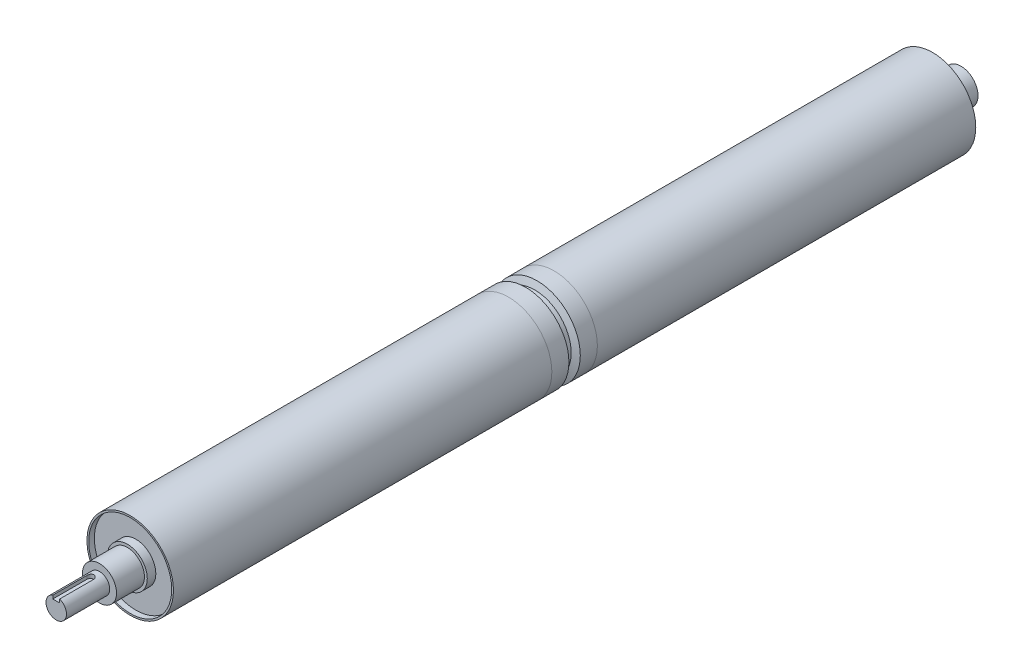
SolidWorks part; units mm, degrees
material "普通碳钢"
ref_plane "前视基准面" through (0, 0, 0) normal (0, 0, 1) x (1, 0, 0)
ref_plane "上视基准面" through (0, 0, 0) normal (0, 1, 0) x (1, 0, 0)
ref_plane "右视基准面" through (0, 0, 0) normal (1, 0, 0) x (0, 0, -1)
sketch "草图1" plane through (0, 0, 0) normal (0, 0, 1) x (1, 0, 0)
  circle A0 centre (0, 0) radius 38
  circle A1 centre (0, 0) radius 36.5
  dimension "D1" = 76
  dimension "D2" = 1.5
extrude "凸台-拉伸1" add sketch "草图1" along normal mid plane 705
sketch "草图2" plane through (0, 0, 352.5) normal (0, 0, 1) x (1, 0, 0)
  circle A1 centre (0, 0) radius 36.5 construction
  circle A2 centre (0, 0) radius 36.5
  circle A3 centre (0, 0) radius 17.5
  dimension "D1" = 35
extrude "凸台-拉伸2" add sketch "草图2" against normal blind 10 from offset 5 separate body offset against normal yes
sketch "草图3" plane through (0, 0, -352.5) normal (0, 0, -1) x (-1, 0, 0)
  circle A1 centre (0, 0) radius 17.5
  circle A2 centre (0, 0) radius 17.5
  circle A3 centre (0, 0) radius 36.5
  circle A4 centre (0, 0) radius 36.5
  dimension "D1" = 0
  dimension "D2" = 0
extrude "凸台-拉伸3" add sketch "草图3" against normal blind 10 from offset 5 separate body offset against normal yes
sketch "草图10" plane through (0, 0, 0) normal (0, 0, 1) x (1, 0, 0)
  circle A0 centre (0, 0) radius 17.5
  dimension "D1" = 35
extrude "凸台-拉伸4" add sketch "草图10" along normal mid plane 755 separate body
sketch "草图11" plane through (0, 0, 377.5) normal (0, 0, 1) x (1, 0, 0)
  circle A1 centre (0, 0) radius 17.5
  circle A2 centre (0, 0) radius 17.5
  dimension "D1" = 0
extrude "凸台-拉伸5" add sketch "草图11" along normal blind 40
sketch "草图15" plane through (0, 0, 417.5) normal (0, 0, 1) x (1, 0, 0)
  circle A0 centre (0, 0) radius 23.9517
  circle A1 centre (0, 0) radius 15
  dimension "D1" = 30
extrude "切除-拉伸2" cut sketch "草图15" against normal blind 62.5
sketch "草图16" plane through (0, 0, -377.5) normal (0, 0, -1) x (-1, 0, 0)
  circle A0 centre (0, 0) radius 15
  circle A1 centre (0, 0) radius 17.5 construction
  circle A2 centre (0, 0) radius 17.5
  dimension "D1" = 30
extrude "切除-拉伸3" cut sketch "草图16" against normal blind 22.5
sketch "草图18" plane through (0, 0, 0) normal (0, 0, 1) x (1, 0, 0)
  circle A0 centre (0, 0) radius 54.9628
  circle A1 centre (0, 0) radius 24.0057
extrude "切除-拉伸4" cut sketch "草图18" against normal mid plane 40
sketch "草图19" plane through (0, 0, 0) normal (0, 1, 0) x (1, 0, 0)
  line L0 (0, 0) -> (-63.5289, 0) construction
  line L1 (-36.5, 30) -> (-36.5, 20)
  line L2 (-36.5, 352.5) -> (-36.5, 20) construction
  line L3 (-36.5, 20) -> (-38, 20)
  line L4 (-38, 20) -> (-38, -20)
  line L5 (-36.5, 30) -> (-17.5, 30)
  line L6 (-17.5, 30) -> (-17.5, -30)
  line L7 (-36.5, -30) -> (-17.5, -30)
  line L8 (-36.5, -20) -> (-38, -20)
  line L9 (-36.5, -30) -> (-36.5, -20)
  line L10 (0, 0) -> (0, 37.0357) construction
  point P14 (-17.5, 0)
  point P16 (-38, 0)
  dimension "D1" = 17.5
  dimension "D2" = 60
revolve "旋转2" add sketch "草图19" angle 360 about L10
sketch "草图17" plane through (0, 0, 0) normal (0, 1, 0) x (1, 0, 0)
  line L0 (118.6374, 0) -> (0, 0) construction
  line L1 (118.6374, 375) -> (38, 375) construction
  line L6 (118.6374, 375) -> (118.6374, 0) construction
  line L12 (0, 0) -> (0, -124.9443) construction
  line L13 (38, -20) -> (38, 20) construction
  line L14 (32, 3) -> (32, -3)
  line L15 (38, 5) -> (32, 3)
  line L16 (38, 5) -> (38, -5)
  line L17 (38, -5) -> (32, -3)
  point P25 (32, 0)
  dimension "D1" = 6
  dimension "D5" = 10
  dimension "D6" = 6
revolve "切除-旋转5" cut sketch "草图17" angle 360 about L12
sketch "草图20" plane through (0, 0, 417.5) normal (0, 0, 1) x (1, 0, 0)
  circle A0 centre (0, 0) radius 25
  circle A1 centre (0, 0) radius 9
  dimension "D1" = 50
  dimension "D2" = 18
extrude "切除-拉伸5" cut sketch "草图20" against normal blind 38
sketch "草图14" plane through (0, 0, 0) normal (0, 1, 0) x (1, 0, 0)
  line L0 (0, -417.5) -> (0, -387.5) construction
  line L1 (-17.5, -417.5) -> (17.5, -417.5) construction
  line L2 (0, -417.5) -> (0, -387.5) construction
  line L3 (-3, -417.5) -> (-3, -387.5)
  line L4 (3, -417.5) -> (3, -387.5)
  arc A0 (-3, -417.5) -> (3, -417.5) centre (0, -417.5) ccw
  arc A1 (3, -387.5) -> (-3, -387.5) centre (0, -387.5) ccw
  point P5 (0, -402.5)
  dimension "D1" = 6
  dimension "D2" = 30
extrude "切除-拉伸1" cut sketch "草图14" against normal blind 3.5 from offset 9
